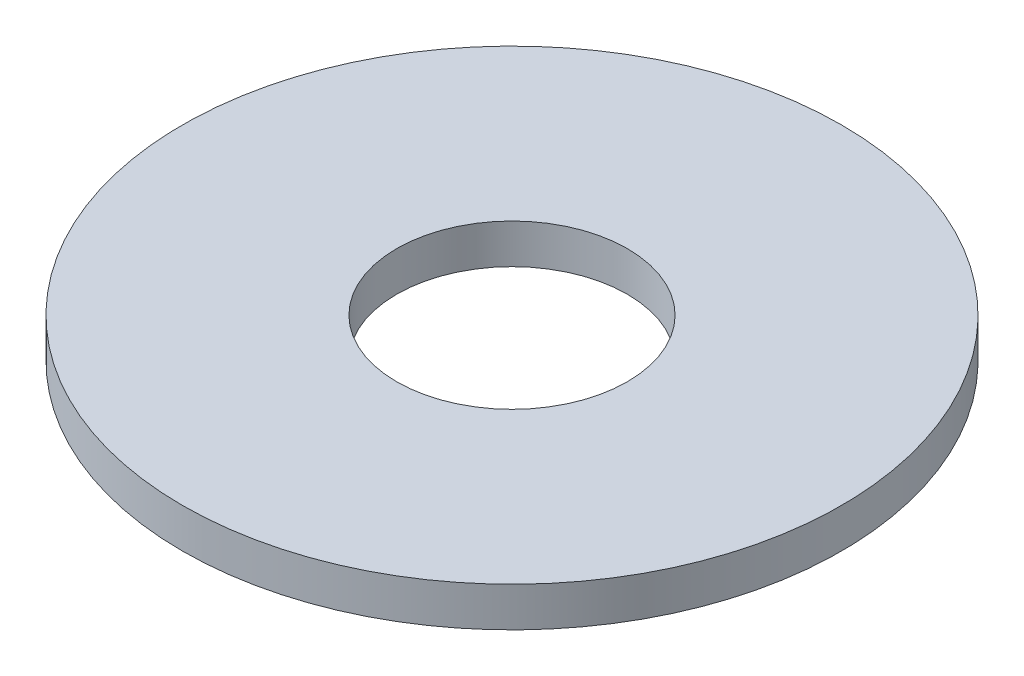
from build123d import *

# Parameters (mm, degrees)
SKETCH1_R           = 25
SKETCH1_R_2         = 8.75
BOSS_EXTRUDE1_DEPTH = 3


with BuildPart() as part:
    # Sketch1 → Boss-Extrude1 (new body)
    with BuildSketch(Plane(origin=(0, 0, 0), x_dir=(1, 0, 0), z_dir=(0, 1, 0))):
        with Locations(Location((0, 0, 0), (0, 0, 270))):
            Circle(SKETCH1_R)
        with Locations(Location((0, 0, 0), (0, 0, 270))):
            Circle(SKETCH1_R_2, mode=Mode.SUBTRACT)
    extrude(amount=BOSS_EXTRUDE1_DEPTH)


solid = part.part
